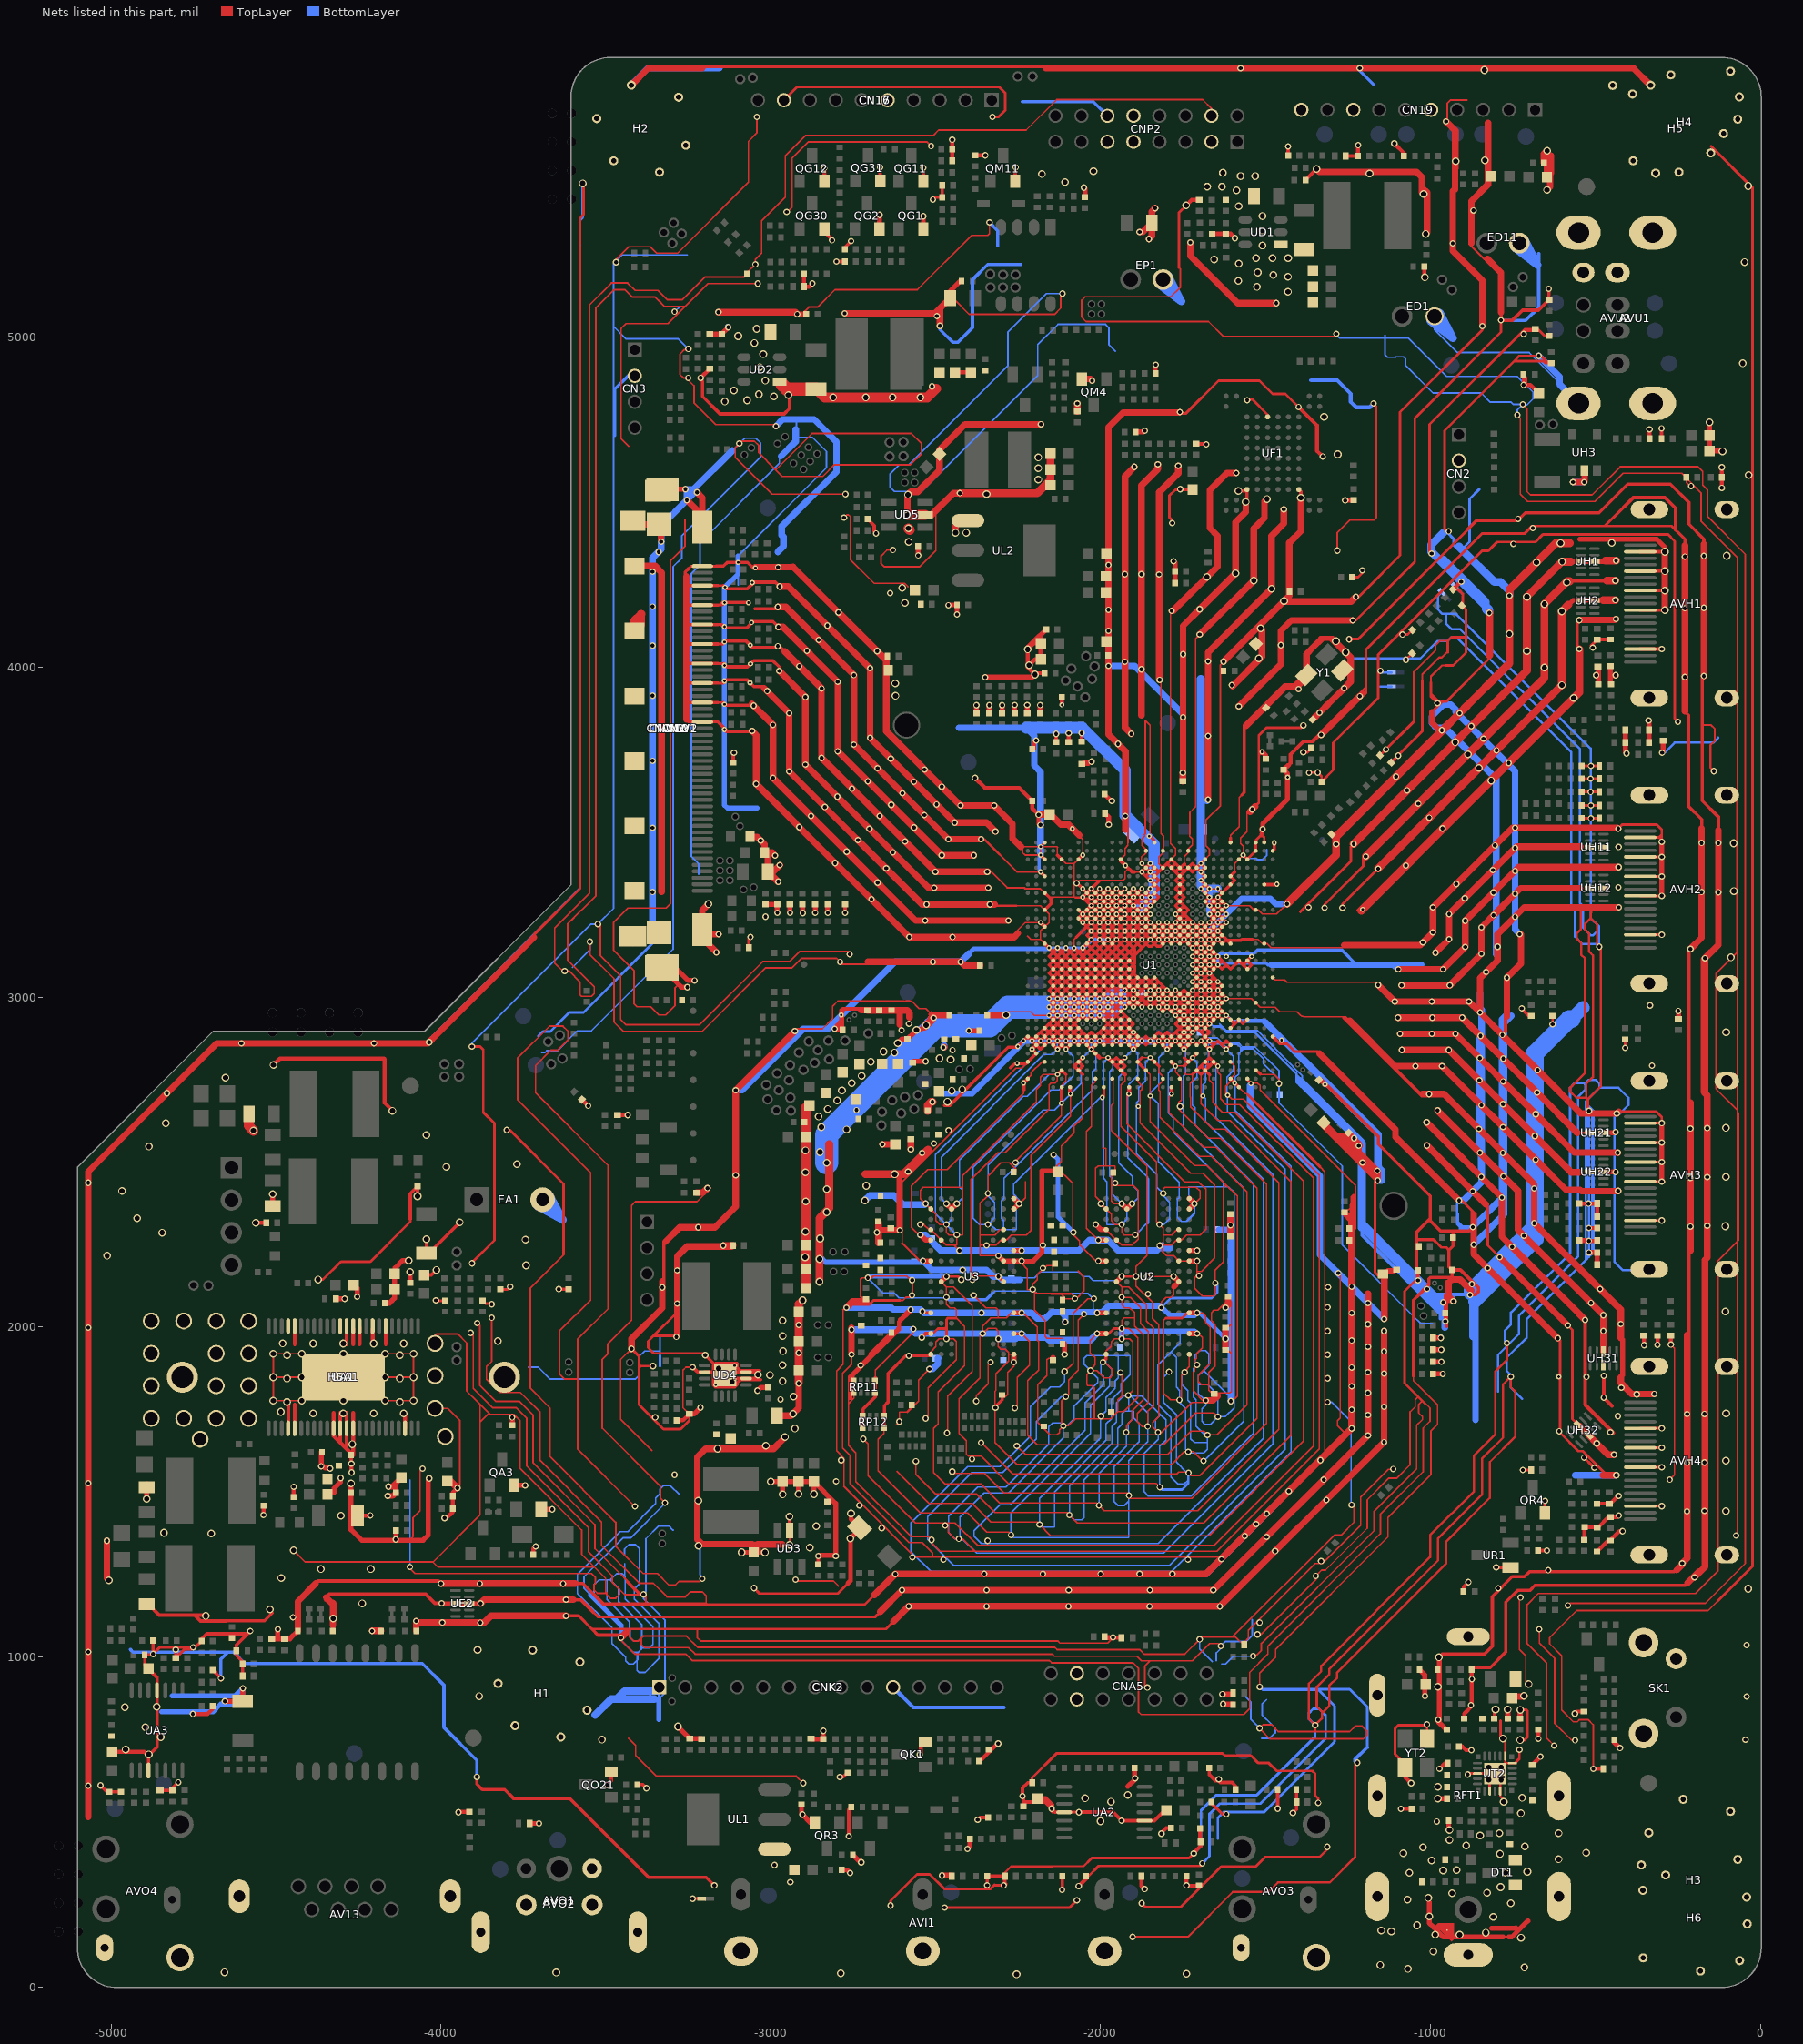
[diagram p0: the nets of this part, all layers, seen from the top]
# Altium PCB MISC86290.PcbDoc (part 20 of 31)
Units mil, origin at the board's own origin, x right, y up, seen from the top; angles counter-clockwise.
Board outline 5104.71 x 5851.49 mil, 2 copper layers (TopLayer, BottomLayer), stack 61.855 mil thick; 1026 components, 667 nets, 4280 pads, 2294 vias.

## Via types
v1: diameter 19.68, hole 11.81, TopLayer to BottomLayer, tented both sides, 1189 vias
v2: diameter 19.68/19.68 (per signal layer), hole 11.81, TopLayer to BottomLayer, tented both sides, 366 vias
v3: diameter 15.75, hole 7.87, TopLayer to BottomLayer, tented both sides, 348 vias
v4: diameter 23.62, hole 15.75, TopLayer to BottomLayer, tented both sides, 309 vias
v5: diameter 15.75/15.75 (per signal layer), hole 7.87, TopLayer to BottomLayer, tented both sides, 59 vias
v6: diameter 24/24 (per signal layer), hole 16, TopLayer to BottomLayer, tented both sides, 23 vias

## Nets (pads, with @x,y where several pads share a name; then routed paths per layer and width w, separated by ;. In a path a pad name is that pad's centre, name@x,y a point inside that pad or via, vN(x,y) a via of type N, cw(c..) or ccw(c..) an arc to the next point about the centre after c; other vN are vias at no path point) (continued)
GND: (continued)
  BottomLayer w3.94: v2(-2706.02,2149.21) -2660.75,2103.94 -2627.28,2103.94 -2611.54,2088.19 -2469.8,2088.19 v2(-2467.83,2090.16) ; v2(-2436.34,2279.13) v2(-2467.83,2310.63) ; v2(-2436.34,2373.62) -2419.61,2390.35 -2419.61,2415.94 -2427.48,2423.82 -2427.48,2506.5 -2234.57,2699.41 -2222.76,2699.41 -2156.81,2765.35 v5(-2131.22,2765.35) ; -2328.07,2101.97 -2321.18,2108.86 -2210.94,2108.86 v2(-2206.02,2113.78) -2194.21,2101.97 -2038.7,2101.97 -2022.95,2086.22 -2022.95,2054.72 v2(-2011.14,2042.91) ; v2(-2310.35,2153.15) -2306.42,2149.21 -2304.76,2149.21 -2242.72,2149.21 -2237.72,2149.21 -2236.72,2149.21 ; -2243.72,2142.99 -2242.94,2142.99 -2236.72,2149.21 ; v2(-2109.57,1864.76) -2109.57,1834.25 -2125.32,1818.5 -2152.87,1818.5 -2212.91,1758.46 -2212.91,1668.9 -2305.43,1576.38 -2403.86,1576.38 -2575.12,1405.12 -2575.12,1319.49 -2515.08,1259.45 -1783.78,1259.45 -1422.56,1620.67 -1422.56,2486.81 -1591.85,2656.1 -1591.85,2756.5 -1582.01,2766.34 -1582.01,2828.35 -1576.1,2834.25 ; v2(-2105.63,1788.98) -2119.41,1788.98 -2195.2,1713.19 -2195.2,1661.02 -2297.56,1558.66 -2391.06,1558.66 -2524.92,1424.8 -2524.92,1355.91 -2446.18,1277.17 -1791.65,1277.17 -1440.28,1628.54 -1440.28,2478.94 -1615.47,2654.13 v5(-1615.47,2702.36) -1617.44,2704.33 -1617.44,2757.48 -1597.76,2777.17 -1597.76,2820.47 v5(-1619.41,2842.13) -1604.65,2856.89 -1584.96,2856.89 -1576.1,2848.03 ; v5(-2105.63,2842.13) -2083.98,2820.47 -2083.98,2761.42 -2126.3,2719.09 -2150.91,2719.09 -2386.14,2483.86 -2386.14,2329.33 -2367.44,2310.63 v2(-2341.85,2310.63) ; v5(-2054.45,2816.54) -2060.35,2810.63 -2060.35,2737.8 v5(-2091.85,2706.3) v5(-2119.41,2678.74) -2140.08,2658.07 -2174.53,2658.07 -2341.85,2490.75 v2(-2341.85,2405.12) -2341.85,2397.24 -2322.17,2377.56 -2322.17,2330.31 v2(-2341.85,2310.63) ; v5(-2028.86,2842.13) -2015.08,2828.35 -2015.08,2783.07 -2024.92,2773.23 -2024.92,2719.09 -2293.62,2450.39 -2293.62,2390.35 -2301.5,2382.48 -2301.5,2329.33 -2294.61,2322.44 -2294.61,2294.88 ; v2(-2005.24,1459.25) -2005.24,1556.69 -1922.56,1639.37 v2(-1922.56,1680.71) -1916.65,1686.61 -1916.65,1707.28 -1899.92,1724.02 ; v5(-1995.39,2695.47) -2002.28,2695.47 -2264.09,2433.66 -2264.09,2402.17 -2247.36,2385.43 v2(-2247.36,2373.62) -2255.24,2365.75 -2255.24,2294.88 -2294.61,2294.88 ; v2(-1993.43,1893.31) -1999.33,1887.4 -1999.33,1857.87 -1991.46,1850 -1991.46,1826.38 -2047.56,1770.28 -2047.56,1686.61 -2273.44,1460.73 -2305.93,1460.73 -2384.17,1382.48 -2384.17,1365.75 -2362.52,1344.09 -1825.12,1344.09 -1507.2,1662.01 -1507.2,2448.43 -1682.4,2623.62 -1682.4,2692.52 v5(-1690.28,2700.39) -1690.28,2733.86 -1681.91,2742.22 -1681.91,2790.45 -1674.53,2797.83 -1674.53,2830.31 ; v2(-1936.34,2153.15) -1948.15,2141.34 -2022.95,2141.34 -2034.76,2153.15 -2052.48,2153.15 -2066.26,2166.93 -2183.39,2166.93 -2201.1,2149.21 -2236.72,2149.21 ; v5(-1926.5,2816.54) v5@-1931.42,2811.61 ; v2(-1904.84,2373.62) -1888.11,2390.35 -1888.11,2413.98 -1903.86,2429.72 -1903.86,2456.3 -1945.2,2497.64 -1945.2,2757.48 -1931.42,2771.26 v5@-1931.42,2811.61 ; v2(-1895,2279.13) -1857.6,2316.54 ; -1857.6,2447.44 -1857.6,2453.35 -1917.64,2513.39 -1917.64,2703.35 v5(-1914.69,2706.3) -1914.69,2734.84 -1887.13,2762.4 -1887.13,2828.35 v5(-1900.91,2842.13) -1900.91,2842.31 -1907.72,2835.49 -1907.72,2835.31 v5@-1931.42,2811.61 ; v5(-1849.72,2816.54) -1863.5,2802.76 -1863.5,2746.65 -1885.16,2725 -1885.16,2686.61 -1892.05,2679.72 -1892.05,2525.2 -1829.06,2462.2 -1829.06,2423.82 v2(-1810.35,2405.12) -1810.35,2398.23 -1790.67,2378.54 -1790.67,2328.35 -1808.39,2310.63 v2(-1822.17,2310.63) ; v2(-1821.18,1514.37) -1821.18,1638.39 -1802.48,1657.09 -1802.48,1718.11 -1818.23,1733.86 ; v5(-1798.54,2842.13) -1824.13,2816.54 -1824.13,2734.84 -1849.72,2709.25 v5(-1849.72,2700.39) -1826.1,2676.77 -1826.1,2502.56 -1762.13,2438.58 -1762.13,2392.32 -1767.05,2387.4 -1767.05,2332.28 -1755.24,2320.47 -1739.49,2320.47 ; v2(-1792.64,1863.78) -1808.39,1848.03 -1808.39,1771.26 -1770.98,1733.86 -1770.98,1590.16 -1738.5,1557.68 v2@-1734.57,1557.68 ; v5(-1772.95,2790.94) -1794.61,2769.29 -1794.61,2649.21 -1779.84,2634.45 -1779.84,2592.13 -1628.27,2440.55 -1628.27,2424.8 ; -1759.17,1987.8 -1759.17,1952.36 -1787.08,1924.46 ; v5(-1747.36,2842.13) -1743.43,2838.19 -1743.43,2832.28 ; v2(-1745.39,1862.8) -1745.61,1862.46 -1753.27,1854.8 -1753.27,1824.41 -1735.55,1806.69 -1735.55,1778.15 -1727.68,1770.28 -1727.68,1661.02 -1715.87,1649.21 -1676.5,1649.21 ; v3@-1743.43,2867.72 -1743.43,2832.28 ; -1734.57,1536.02 -1746.38,1524.21 -1766.06,1524.21 -1786.73,1544.88 -1786.73,1725.98 -1827.09,1766.34 -1827.09,1884.45 -1787.08,1924.46 ; v2(-1734.57,1621.65) v2@-1735.06,1621.16 ; v5(-1721.77,2816.54) -1707.99,2802.76 -1707.99,2756.5 -1721.77,2742.72 -1721.77,2672.83 -1713.9,2664.96 -1713.9,2611.81 -1536.73,2434.65 -1536.73,1677.76 -1726.69,1487.8 -1855.63,1487.8 -1868.43,1500.59 -1868.43,1616.73 -1826.1,1659.06 v2(-1826.1,1680.71) -1833.98,1688.58 -1833.98,1718.11 -1818.23,1733.86 ; -1715.87,2344.09 v2(-1715.87,2373.62) -1715.87,2380.51 -1732.6,2397.24 -1732.6,2424.8 -1628.27,2424.8 ; v2(-1707.99,1885.43) v2@-1708.21,1885.22 ; v2(-1688.31,1594.09) -1686.34,1594.09 -1566.26,1714.17 -1566.26,2420.87 -1750.32,2604.92 -1750.32,2660.04 v2(-1759.17,2668.9) -1750.32,2677.76 -1750.32,2759.45 -1743.43,2766.34 -1743.43,2832.28 ; v2(-1676.5,1672.83) v2@-1676.5,1664.96 ; -1674.53,2857.87 -1674.53,2830.31 ; v5(-1670.59,2842.13) -1674.53,2838.19 -1674.53,2830.31 ; v3@-1670.59,2861.81 v3(-1670.59,2867.72) ; v5(-1645,2790.94) -1645,2789.96 -1649.92,2785.04 -1649.92,2634.45 -1477.68,2462.2 -1477.68,1646.26 -1809.37,1314.57 -2376.3,1314.57 -2419.27,1357.53 -2430.43,1357.53 v2(-2430.43,1357.87) ; -1605.63,1785.92 -1687.87,1868.15 ; -1560.3,2843.03 -1567.32,2843.03 -1571.98,2838.38 ; v2(-2467.83,2310.63) -2452.09,2326.38 -2452.09,2357.87 v2(-2467.83,2373.62) -2483.58,2389.37 -2483.58,2514.37 -2172.56,2825.39 -2147.95,2825.39 v5(-2131.22,2842.13) -2131.22,2859.21 -2139.72,2867.72 v3(-2156.81,2867.72) -2501.3,2523.23 -2501.3,2344.09 v2(-2467.83,2310.63) ; v2(-2430.43,1357.87) -2442.24,1357.87 -2460.94,1376.57 -2460.94,1425.79 -2372.36,1514.37 -2287.72,1514.37 -2157.8,1644.29 -2157.8,1697.44 -2145.98,1709.25 -2122.36,1709.25 v2(-2113.5,1700.39) ; v2(-2430.43,1357.87) -2430.43,1358.86 -2426.5,1362.8 -2426.5,1423.82 -2353.66,1496.65 -2279.84,1496.65 -2113.5,1662.99 v2(-2113.5,1700.39) ; v2(-2341.85,2310.63) -2333.98,2310.63 -2318.23,2294.88 -2294.61,2294.88 ; v2(-2113.5,1700.39) -2101.69,1700.39 -2081.02,1721.06 -2081.02,1760.43 -2009.17,1832.28 -2009.17,1844.09 -2032.4,1867.32 v2(-2030.83,1867.72) -2050.51,1887.4 -2050.51,1905.12 -2042.64,1912.99 -1983.58,1912.99 ; -1983.58,1912.99 -1946.18,1912.99 ; -1983.58,1912.99 -1983.58,1889.37 -1965.87,1871.65 -1965.87,1854.92 -1973.74,1847.05 -1973.74,1820.47 -2030.83,1763.39 -2030.83,1677.76 -2271.97,1436.61 v2(-2271.97,1369.69) -2264.09,1361.81 -1915.67,1361.81 v2@-1915.67,1488.78 ; -1946.18,1912.99 -1910.75,1912.99 -1910.75,1855.91 -1938.31,1828.35 -1938.31,1808.66 -1967.83,1779.13 -1967.83,1722.05 -1983.58,1706.3 -1983.58,1656.1 -2140.08,1499.61 -2140.08,1393.31 -2178.46,1393.31 -2185.35,1400.2 v2(-2185.35,1401.18) -2185.35,1479.92 -2001.3,1663.98 -2001.3,1727.95 v2(-1999.33,1729.92) -1983.58,1745.67 -1983.58,1787.01 -1956.02,1814.57 -1956.02,1836.22 -1946.18,1846.06 -1946.18,1912.99 ; v2@-1916.65,1790.94 -1916.65,1787.01 -1914.69,1785.04 -1914.69,1745.67 ; v2@-1916.65,1790.94 -1931.42,1790.94 -1952.09,1770.28 -1952.09,1712.2 -1965.87,1698.43 -1965.87,1647.27 -2094.8,1519.29 v2(-2094.8,1429.72) -2081.02,1415.94 -2057.4,1415.94 -2050.51,1422.83 -2050.51,1537.01 -1948.15,1639.37 -1948.15,1692.52 -1936.34,1704.33 -1936.34,1736.81 -1927.48,1745.67 -1914.69,1745.67 ; v2@-1916.65,1790.94 v2(-1916.65,1792.91) -1908.78,1790.94 -1857.6,1739.76 v2(-1857.6,1698.43) -1857.6,1653.15 -1915.67,1595.08 v2@-1915.67,1488.78 ; v2@-1916.65,1790.94 -1875.32,1790.94 -1818.23,1733.86 ; v2@-1915.67,1488.78 v2(-1914.69,1488.78) -1914.69,1472.05 -1928.46,1458.27 -1947.17,1458.27 -1959.96,1471.06 -1959.96,1576.38 -1883.19,1653.15 -1883.19,1707.28 -1899.92,1724.02 ; -1914.69,1745.67 -1899.92,1745.67 -1899.92,1724.02 ; -1787.08,1924.46 -1770.98,1908.36 -1770.98,1817.52 -1761.14,1807.68 v2(-1761.14,1779.13) -1761.14,1771.26 -1743.43,1753.54 -1743.43,1629.53 v2@-1735.06,1621.16 ; v2@-1735.06,1621.16 -1731.61,1617.72 -1688.31,1617.72 -1676.5,1629.53 -1676.5,1649.21 ; v2@-1734.57,1557.68 v2(-1733.58,1557.68) -1734.57,1556.69 v2@-1734.57,1557.68 ; v2@-1708.21,1885.22 -1719.8,1873.62 -1719.8,1787.99 -1710.94,1779.13 -1710.94,1699.41 v2@-1676.5,1664.96 ; v2@-1708.21,1885.22 -1713.9,1890.9 -1713.9,1914.96 -1700.12,1928.74 -1682.4,1928.74 -1672.56,1918.9 -1672.56,1883.46 -1687.87,1868.15 ; -1704.06,1824.41 -1704.06,1797.83 -1688.31,1782.09 v2(-1681.42,1777.17) -1681.42,1764.37 -1693.23,1752.56 -1693.23,1714.17 -1684.37,1705.31 -1667.64,1705.31 v2(-1645,1727.95) ; -1704.06,1824.41 -1675.51,1824.41 -1645,1793.9 v2(-1645,1727.95) ; -1704.06,1824.41 -1704.06,1851.97 -1687.87,1868.15 ; -1676.5,1649.21 v2@-1676.5,1664.96 ; v2(-1645,1727.95) -1622.36,1727.95 -1595.79,1754.53 -1595.79,2408.07 -1612.52,2424.8 -1628.27,2424.8 ; -1576.1,2834.25 -1571.98,2838.38 ; -1576.1,2834.25 -1576.1,2848.03 ; -1576.1,2848.03 -1576.1,2842.5 -1571.98,2838.38 ; -1991.46,2450.39 -1991.46,2802.76 v5(-1977.68,2816.54) -1962.91,2801.77 -1962.91,2783.07 -1972.76,2773.23 -1972.76,2458.27 -1963.9,2449.41 -1963.9,2401.18 v2(-1936.34,2373.62) -1920.59,2357.87 -1920.59,2326.38 v2(-1936.34,2310.63) -1981.61,2310.63 -1981.61,2440.55 -1991.46,2450.39
  BottomLayer w4: -3402.82,1013.16 -3402.82,992.13 -3405.84,989.1 -3416.68,978.26 -3430.63,978.26 -3440.5,988.13 ; -3276.73,1490.73 -3305,1519 -3326,1519 -3336.8,1508.2 -3336.8,1494.2 -3349,1482 -3349,1464.43 -3433.27,1380.16 -3456.27,1380.16 -3586,1250.42 -3586,1192 -3482,1088 -3482,1040.75 -3440.5,999.25 ; -3440.5,988.13 -3440.5,999.25 ; -3440.5,988.13 -3440.5,999.25
  BottomLayer w4.92: v3(-1568.23,3430.71) -1557.97,3420.45 -1528.48,3420.45 -1524.5,3416.47 -1509.6,3416.47 -1497,3429.07 -1497,3448
  BottomLayer w5: v1(-4094,1273) -4094,1536.22 ; -4035.91,2873.58 -3579.11,3330.38 -3579.11,3359 ; v1(-3906.34,2849.93) -3906.34,2860.32 -3545.24,3221.42 v1(-3524.48,3221.42) -3476.61,3269.28 -3476.61,5033 ; -3735.25,1878 -3705.25,1878 -3669.25,1842 -3411.29,1842 -3399.5,1853.78 -3399.5,1909.82 -3382.32,1927 -3335.84,1927 ; -3695,2831.5 -3685.5,2831.5 -3679.5,2837.5 -3647.12,2837.5 -3587.6,2897.01 -3544.44,2897.01 -3296.11,3145.34 -3296.11,4305.72 -3269.75,4332.09 ; v1@-3628,3082.32 v1(-3624.82,3079.14) ; -3601.36,3090.14 -3548.82,3142.68 v1(-3548.82,3168.12) ; -3546,1187.87 -3566.5,1208.37 -3566.5,1242.35 -3448.19,1360.66 -3425.19,1360.66 -3321,1464.85 v1(-3321,1467) ; -3536.34,1180.31 -3536.34,1218 -3520.84,1233.5 -3487,1233.5 ; -3499,1233.5 -3496.82,1231.32 -3496.82,1174.05 -3428.28,1105.5 -3428.28,1064 ; v1(-3469,5228) v1@-3468.5,5228 ; v1(-3454.25,1058) -3454.25,1050.22 -3417.18,1013.16 -3402.82,1013.16 ; -3444,1309 -3444,1326.5 -3429.84,1340.66 -3411.16,1340.66 -3398.75,1328.25 -3398.75,1221.39 -3414,1206.14 -3414,1176.08 -3339.25,1101.32 -3339.25,994.75 ; -3443,1244.96 -3443,1282 ; -3427.28,1082.77 -3427.28,1059.25 -3416.18,1048.16 -3401.82,1048.16 -3392.84,1057.13 ; -3386.59,905.59 -3377.19,896.19 -3353,872 -3339.87,872 -3320.72,891.15 -3320.72,1111.08 -3386.09,1176.45 v1(-3386.09,1189.34) -3378.75,1196.68 -3378.75,1358.25 -3340,1397 -3309.5,1397 -3296.5,1384 ; CNK2.1@-3353.59,914.59 -3339.87,900.87 -3339.87,873.51 ; -3339.25,1070 -3339.25,994.75 ; -3335.84,1912.5 -3335.84,1973.66 ; v1(-3292,5078) -3275.16,5094.84 ; -3269.75,4397.61 -3269.75,4332.09 ; -3252.5,5249.84 -3451.16,5249.84 -3476.61,5224.39 -3476.61,5033 ; v1(-3250.5,4877.5) v1@-3250,4877.5 ; v1(-3250,4965) -3280.5,4995.5 -3439.11,4995.5 -3476.61,5033 ; -3219,3372 -3219,3404.58 -3241.11,3426.69 -3241.11,4282.94 -3214.75,4309.3 -3214.75,4377.61 -2974,4618.36 -2974,4639 ; v4@-3215,1331 -3215,1249.53 -3208,1242.53 v1(-3208,1237) ; v4@-3196,3289 v4(-3189,3282) ; v1(-3192,2421) v1@-3192,2422 ; -3116.5,4657.2 -3079.2,4694.5 -3045.5,4694.5 -3031,4680 -3031,4637.77 -3269.75,4399.02 -3269.75,4332.09 ; -3099.25,4250 -3099.25,4337.54 -2831.5,4605.29 -2831.5,4654.11 -2873.89,4696.5 -2920,4696.5 ; -2924.41,4756.41 -2922,4754 -2922,4678 ; v2@-2237.66,1978.09 v2@-2237.6,1978.03 ; -2237.25,5717.46 -2045.62,5717.46 -2043.12,5714.96 ; v1(-2116.25,5133) -2165,5133 -2281,5017 -2281,4914.49 -2581.99,4613.5 -2611.5,4613.5 -2639,4586 -2639,4547 -2625,4533 -2542.25,4533 -2191,4884.25 -2191,4978 -2129.5,5039.5 -1985,5039.5 -1975.34,5029.84 -1975.34,4978.32 -1955.18,4958.16 ; v5(-2054.45,2816.54) v5(-2028.86,2842.13) v3(-2028.86,2867.72) ; CNP2.12@-1999.9,5671.74 CNP2.12@-1994.9,5671.74 ; v3(-1926.5,2867.72) v3@-1925.81,2867.72 ; v1(-1700,1053) -1700,1024 -1661.66,985.66 ; -1689.1,2885.8 -1679.6,2876.3 -1646.67,2876.3 -1631.17,2860.8 -1581.75,2860.8 -1569.75,2848.8 -1532.19,2848.8 -1459.22,2775.84 v2(-1459.22,2737.78) ; -1677.73,2931 -1656.73,2910 -1636.1,2910 ; v3(-1670.59,3251.57) v3@-1670.59,3252.21 ; -1649.5,989 -1649.5,1012.02 -1636,1025.52 v1(-1636,1033) ; -1639.6,2918.9 -1616.84,2896.14 -1613,2896.14 ; v1@-1637,1034 v1(-1636,1033) ; -1633.5,978.5 -1621.5,978.5 -1598,1002 v1(-1538,1002) ; -1630.7,2910 -1636.1,2910 ; -1624.63,2903.94 -1624.63,2898.53 ; -1576.1,2848.03 -1576.01,2848.03 -1571.01,2843.03 -1537.22,2843.03 -1505.9,2811.71 -1505.9,2797.35 -1459.22,2750.67 v2(-1459.22,2737.78) ; -1560.5,878.5 -1545.34,863.34 -1545.34,811.2 v1(-1518.23,784.09) v1@-1518.23,782.7 ; -1540.5,1112.69 -1540.5,1065.5 -1559.67,1046.33 -1622.67,1046.33 v1(-1636,1033) ; -1531.92,2894.29 -1536.16,2898.53 -1539,2898.53 ; -1512.5,753 -1487.47,753 -1470.66,769.82 -1470.66,784.18 -1480.82,794.34 -1481.34,794.34 -1510.66,823.66 -1510.66,856.84 -1497.5,870 ; -1389,2747.81 -1389,2760.81 -1417.29,2789.1 -1417.29,2790.49 -1525.33,2898.53 -1539,2898.53 ; v1(-1331.84,1290.34) v1@-1328.19,1294 ; v2(-1312.32,1772.24) -1300.24,1772.24 -1240.97,1712.97 -1240.97,1459 v1(-1239.35,1460.62) ; v1@-1287,5010 -1275,4998 -1067,4998 -951,4882 -737.47,4882 -688.66,4833.18 -688.66,4814.34 -708,4795 v1@-722.13,4795 ; v1@-1286,5010.5 v1(-1286,5011) ; -1206.37,2514.37 -1206.37,2324.84 -1202.37,2320.84 -970.5,2088.96 -970.5,2084.9 v1@-970.5,2073.4 ; -1138,5007 -1138,4947 -1131,4940 -1105.53,4940 -1104.18,4941.34 -1081.73,4941.34 -1075.34,4934.95 -1075.34,4914.67 -992.17,4831.5 -847.02,4831.5 -819.17,4803.66 -755.66,4803.66 -748.85,4796.85 v1(-720.28,4796.85) v1@-722.13,4795 ; -1037,2017.57 -1044.97,2025.54 ; -995,2011 -1030.43,2011 -1044.97,2025.54 ; ED1.2@-988.04,5064 -988.04,5024.04 -918,4954 -701,4954 -609,4862 -551.16,4804.16 AVU2.9@-551.16,4800.38 ; v1(-913.55,2383.45) -919.34,2377.66 -919.34,2322.82 -897.53,2301 -895.53,2303 v1(-872,2303) ; v1(-737.11,4764.63) -737.11,4780.03 v1@-722.13,4795 ; v1(-727.5,1180) v1@-726.5,1180 ; v1@-301,4055 v1(-299,4055) ; -3402.82,1013.16 -3392.66,1023.32 -3392.66,1027 ; -3402.82,1013.16 -3405.84,1010.13 -3405.84,989.1 -3405.84,959.34 -3399,952.5 -3381.5,952.5 -3339.25,994.75 ; -3392.84,1057.13 -3392.84,1038.32 -3392.66,1038.13 -3392.66,1027 ; -3392.84,1057.13 -3391,1058.97 -3391,1096.51 -3461.34,1166.85 -3461.34,1207.34 -3487,1233 -3468,1252 -3450,1252 -3441.34,1243.34 -3441.34,1175.13 -3357.25,1091.04 -3357.25,1037.75 -3368,1027 -3392.66,1027 ; -1636.1,2910 -1624.63,2898.53 ; -1624.63,2898.53 -1539,2898.53 ; v2(-1459.22,2737.78) -1459.22,2679.15 -1267.67,2487.6 -1267.67,2248.24 -1044.97,2025.54
  BottomLayer w5.91: -1739.49,2320.47 -1715.87,2344.09
  BottomLayer w6: -920,2333 -920,2377 v1(-913.55,2383.45)
  BottomLayer w7: -1656.73,2910.84 -1636.95,2910.84 ; -1624.1,2899.53 -1618.04,2893.48 -1531.92,2893.48 ; -1532.3,2893.48 -1406.32,2767.5 -1406.32,2765.13 ; -1392.73,2728.53 -1406.32,2742.12 -1406.32,2765.13 ; -1389,2747.81 -1406.32,2765.13 ; -1387.59,2746.41 -1387.59,2749.16 ; v1@-1262.84,4505.84 v1(-1258.63,4505.84) ; -1237,4027 -1031,4027 -979,4079 -948.65,4079 -936.65,4091 -922,4091 -573,3742 -573,3277.19 -562.34,3266.53 -562.34,3183.4 -540.44,3161.5 -489.5,3161.5 v1@-489,3162 ; -1231.66,683.34 -1231.16,683.84 -1190.28,724.72 ; -1152.42,3942 RO17.JP_2K@-1118.44,3942 ; v1(-1151.76,3989.5) -1148,3985.74 -1148,3984 RO18.JP_2K@-1118.44,3984 ; RO35.JP_2K@-965.91,4227.91 -978,4215.82 -978,4176 -964,4162 -923.06,4162 -514.34,3753.28 -514.34,3239.4 -489,3214.06 -489,3201 ; -953,4161 -953,4133.06 -934.94,4115 -910,4115 -547,3752 -547,3285.13 -538.34,3276.47 -538.34,3211.4 -513.94,3187 -508,3187 -494,3201 -489,3201 ; -920,2333 -918.5,2331.5 ; -796,1804.06 -796,1914.53 -732.54,1977.99 -732.54,2033.66 -553,2213.21 -553,2696.97 -530.99,2718.99 -530.99,2738.01 -520,2749 -500,2749 -487.95,2736.95 -487.95,2725.34 ; v1(-768.38,1951.12) -775.34,1958.07 -775.34,1988.6 -756.54,2007.4 -756.54,2043.6 -577,2223.15 -577,2724.94 -562.6,2739.34 -536.14,2739.34 -530.99,2734.18 ; -722.03,1781.97 -757,1816.94 v1(-757,1849) -754,1852 -769.34,1867.34 -769.34,1907.25 -708.54,1968.05 -708.54,2023.72 -529,2203.26 ; v1@-523.23,2218.34 -529,2212.56 ; v1(-489,3153) v1@-489,3162 ; AVH3.20@-367,2173 -418,2173 -443,2198 -443,2640.01 v1(-435.5,2647.5) -425.5,2647.5 -400,2673 -400,2695 -430.34,2725.34 -487.95,2725.34 ; v1(-298,3741) -290.69,3741 -260.34,3771.34 -143.16,3771.34 -127.5,3787 ; -529,2203.26 -519.69,2212.58 ; -529,2203.26 -529,2212.56 ; -529,2212.56 -529,2684.29 -523.23,2690.06 ; v1@-523.23,2658.54 v1(-519.69,2655) -519.69,2417.19 ; v1@-523.23,2658.54 -523.23,2420.73 -519.69,2417.19 ; v1@-523.23,2658.54 -523.23,2672.73 ; -523.23,2672.73 -523.23,2690.06 ; -523.23,2672.73 -509.5,2659 ; -523.23,2690.06 -512.48,2700.81 ; -519.69,2212.58 v1(-519.69,2226) -519.69,2376.69 -519.69,2417.19 ; -519.69,2212.58 -509.5,2222.76 ; -519.69,2417.19 -509.5,2407 ; -512.48,2700.81 -491.77,2721.52 ; -512.48,2700.81 -491.77,2721.52 ; -509.5,2222.76 -509.5,2407 ; -509.5,2222.76 -505.5,2226.76 -505.5,2403 ; -509.5,2407 -509.5,2659 ; -509.5,2407 -505.5,2403 ; -509.5,2659 -505.5,2655 -505.5,2403 ; -491.77,2721.52 -487.99,2725.3 ; -491.77,2721.52 -487.99,2725.3 ; v1@-489,3162 -489,3201 ; -487.99,2725.3 -487.95,2725.34
  BottomLayer w7.87: v2(-1821.18,1514.37) -1814.29,1507.48 -1753.27,1507.48 -1734.57,1526.18 -1734.57,1536.02 v2@-1734.57,1556.69 ; v2(-1816.26,2058.66) -1787.72,2087.2 -1663.7,2087.2 -1646.97,2103.94 -1646.97,2129.53 -1650.91,2133.46 v2(-1652.87,2133.46)
  BottomLayer w8: v1@-4016,2082 v1(-4015,2081) ; -3705,2882 -3691,2896 -3668.52,2896 -3611.01,2953.51 -3567.84,2953.51 -3358.61,3162.75 -3358.61,3223.74 ; -3579.11,3359 -3579.11,5354.5 -3570.25,5363.36 v4(-3570.25,5467) ; -3336.5,1881.5 -3336.5,1914 ; v3@-3140.47,4243.97 v3(-3139,4242.5) ; v1@-2151,537.52 v1(-2148.66,539.86) ; v5(-1798.54,2842.13) v3(-1798.54,2867.72) ; v1(-1718,404) -1696.04,425.96 -1696.04,534.19 -1649.23,581 -1526.54,581 -1350,757.54 v1(-1350,793) -1369.16,812.16 -1369.16,829.49 -1355.8,842.84 -1338.34,842.84 -1318,822.5 -1318,752.77 -1515.77,555 -1638.46,555 -1670,523.46 -1670,396 v1(-1692,374) ; -1645,449.74 -1645,511.69 -1627.69,529 -1505,529 -1291.32,742.68 -1291.32,851.32 -1340.04,900.04 -1509.04,900.04 -1510.84,901.84 ; v1(-1518,909) -1510.84,901.84 ; v1@-1401.98,3934 v1(-1400,3934) ; -1231.16,683.84 -1231.16,689.16 -1192.16,728.16 -1192.16,848.8 -1245.2,901.84 -1510.84,901.84 ; v1(-1206.84,4294.01) v1@-1205.33,4292.5 ; -1165.63,2483.5 -1165.63,2477.92 v1(-1161.28,2473.58) ; v1@-1015.87,799.87 v1(-1011,795) ; v1(-996.91,4345) v1@-996.91,4349.3 ; v1(-979,3891) v1@-978,3892 ; -960.38,4408.72 -949.46,4408.72 -930.42,4389.68 -930.42,4370.93 -912.75,4353.25 ; -905.09,4356.91 -881.66,4380.34 -881.66,4510.16 -852,4539.82 ; v1@-750.84,4374.16 v1(-748.89,4374.16) ; v1@-698.5,4422 v1(-690,4422)
  BottomLayer w9.84: v2(-2467.83,2090.16) -2459.96,2082.28 -2347.76,2082.28 -2328.07,2101.97 ; -1857.6,2316.54 -1857.6,2447.44 ; v3(-1619.41,2944.49) -1602.09,2927.17 ; -1512.62,2927.17 -1602.09,2927.17 ; -1506.42,2929.53 -1582.79,2929.53 -1585.16,2927.17 -1602.09,2927.17
  BottomLayer w10: -4941.25,1022 -4933.25,1014 -4646.06,1014 ; v1(-4796.5,619.5) v1@-4793.32,622.68 ; v1(-4667,935) -4667,993.06 -4646.06,1014 ; v1@-3889,636 v1(-3891,636) -3891,686.17 -3991,786.17 -3991,914.46 -4056.54,980 -4594,980 -4628,1014 -4646.06,1014 ; -3473.11,4703.11 -3473.11,4843 -3432.24,4883.87 CN3.2@-3412.5,4883.87 ; -3156.25,5815.96 -3151.25,5820.96 ; -3150,5820.96 -1225.96,5820.96 ; v1@-2790.69,634.53 v1(-2790.69,635.88) ; v1(-2487.25,5035) -2487.25,5024.25 -2448,4985 -2433,4985 -2388.7,5029.3 -2388.7,5174.72 ; -2388.7,5106.5 -2388.7,5174.72 ; v1(-2337.25,5348.75) -2312,5323.5 -2312,5277.5 ; -2241.74,5220.74 -2342.67,5220.74 -2388.7,5174.72 ; -2237.25,5714.96 -2043.12,5714.96 -2022.69,5714.96 CNP2.12@-1979.47,5671.74 CNP2.12@-1994.9,5671.74 ; v3(-2182.4,3379.53) -2186.72,3383.85 -2186.72,3426.39 v3(-2182.4,3430.71) ; v3@-2130.77,3149.21 v3@-2129.21,3147.65 ; v3@-2105.21,3149.21 v3@-2104,3148 ; v1(-1619.5,523) v1@-1617,525.5 ; -1540.62,2929.61 -1521.89,2929.61 ; -1467.55,3098.03 -1493.6,3098.03 -1498.57,3102.99 -1640.04,3102.99 v3(-1645,3098.03) -1645,3125.15 -1637.71,3132.44 -1535.69,3132.44 -1524.94,3143.19 -1269.24,3143.19 -1224.09,3098.03 -1219.93,3098.03 ; -1309,2735.5 -1165.63,2592.13 -1165.63,2546 ; -1227.2,5820.96 -1173.25,5767 ; v1@-1161.28,2444.78 v1(-1160.5,2444) ; v1(-1038,2141.5) v1@-1038,2143 ; -970.5,2024.4 -970.5,2059.9 -970.5,2081.5 -970.5,2091.9 ; -918.5,2341.44 -918.5,2331.5 -918.5,2311.37 -905.29,2298.16 ; v1(-786.25,5052) -711,5052 -672,5091 -672,5254.5 ; v1@-725,2967.5 v1(-723.5,2966) ; v1(-647.5,1322.5) v1@-644.5,1322.5
  BottomLayer w11.81: v2(-2706.02,2149.21) -2702.09,2153.15 -2569.72,2153.15 ; v2(-2571.72,2142.03) -2569.72,2142.03 -2569.72,2153.15 ; v2(-2467.83,2153.15) -2569.72,2153.15 ; v5(-1900.91,2842.13) v3(-1900.91,2867.72) ; v2(-1707.99,2042.91) -1700.12,2042.91 v2(-1621.38,1964.17)
  BottomLayer w12: CNK2.10@-2629.46,908 -2567.96,846.5 -2293.5,846.5 ; v1(-2196,3778) v1@-2196,3779 ; v3(-2117.5,3886) v3@-2117.5,3892.75 ; v3(-1875.32,3302.76) v3(-1849.72,3328.35) ; -1665.05,2861.42 -1638.41,2861.42 -1622.34,2845.35 v5@-1619.41,2845.35 ; -1362.5,4870 -1282.83,4870 -1241.78,4828.95 -1241.78,4804.28 -1226,4788.5 -1184.5,4788.5 v1(-1173,4800) ; -1202.37,2320.84 -1202.37,2316.77 ; -983.55,2098.66 -893.34,2098.66 ; -970.5,2041.4 -1207.17,2278.07 -1207.17,2321.57 -1202.37,2316.77 ; -970.5,2059.9 -961.1,2050.5 ; v1@-958.6,2073 -970.5,2084.9 -1202.37,2316.77 ; -958.6,2091.5 -957,2091.5 ; AVU2.9@-551.16,4800.38 AVU2.9@-524,4773.21 ; v1@-520,2377 -519.69,2376.69 v1@-519,2376
  BottomLayer w14: -2399.15,3132.36 -2384.47,3147.03 -2055.22,3147.03 -2028.86,3173.4 v3(-2028.86,3174.8) ; v2(-2143.03,2522.24) -2129.72,2508.94 -2129.72,2333.74 v2(-2082.99,2287.01)
  BottomLayer w15: -4846.88,833.38 -4691.12,833.38 -4667.5,857 -4609.6,857 -4600.5,866.1 v1(-4600.5,905) ; -4815,882 -4623.5,882 v1(-4600.5,905) ; v1@-4655.5,865.5 v1(-4655,865.5) ; v1@-4600.5,906 v1(-4600.5,905) ; v4(-4272.45,1525.51) v4@-4272.24,1525.3 ; -4145.53,2083.53 -4144.53,2083.53 ; -3546,1187.87 -3454.25,1096.12 v1(-3454.25,1058) ; -3339.87,809.68 -3339.87,872 -3339.87,873.51 ; -3141.11,3596 -3141.11,3604 ; v1@-3131.27,5033.11 v1(-3128.92,5030.76) ; -3099.25,4337.54 -3099.25,4283.38 -3141.11,4241.52 -3141.11,3604 ; -3041,3573.5 -3132,3573.5 -3141.11,3582.61 -3141.11,3604 ; v1@-2805.43,2905.26 v1@-2805.43,2908.74 ; v4(-2759,1359) v4@-2759,1359.43 ; v1@-2402,2900 v1(-2400.03,2898.03) ; v1@-2188.72,3553 v1(-2188,3553) ; -2139.72,2867.72 -2117.44,2867.72 ; v3(-2028.86,3174.8) v3(-1977.68,3174.8) ; v3@-1671.25,2867.62 -1665.05,2861.42 ; v1@-1233.62,2575.53 -1231.9,2573.81 v1(-1231.9,2572.4) ; v1(-969,1967) v1@-969,1971